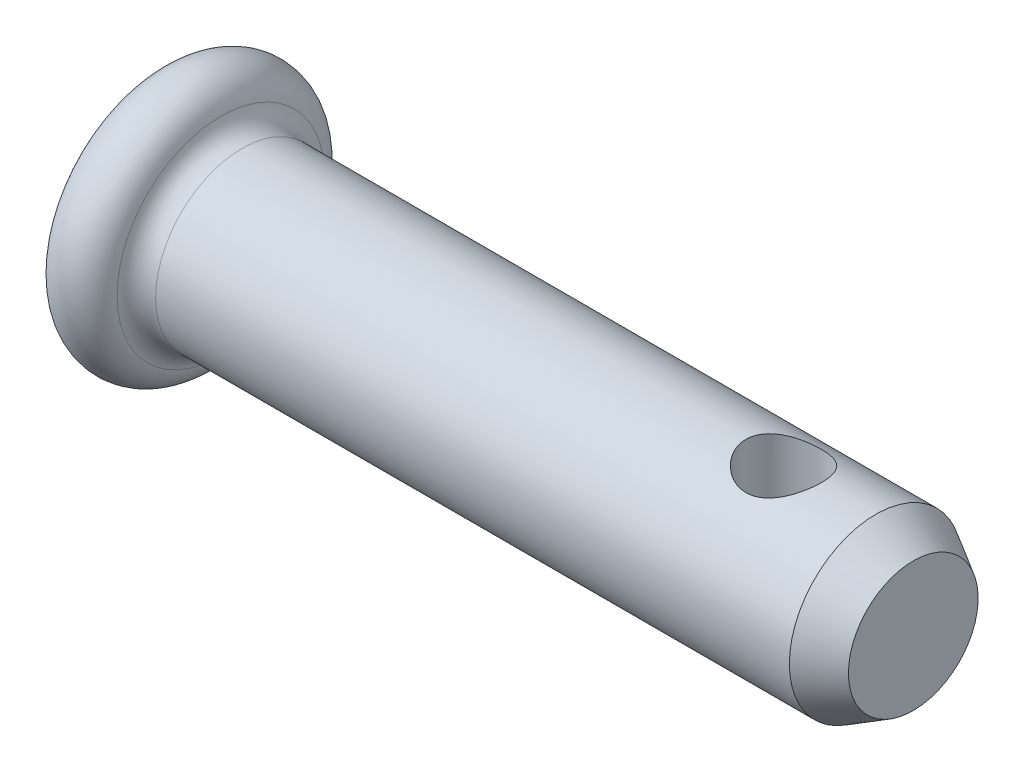
SolidWorks part; units mm, degrees
material "35钢"
ref_plane "前视" through (0, 0, 0) normal (0, 0, 1) x (1, 0, 0)
ref_plane "上视" through (0, 0, 0) normal (0, 1, 0) x (1, 0, 0)
ref_plane "右视" through (0, 0, 0) normal (1, 0, 0) x (0, 0, -1)
sketch "尺寸草图" plane through (0, 0, 0) normal (0, 0, 1) x (1, 0, 0)
  line L0 (0, 6) -> (0, 0)
  line L1 (0, 0) -> (16, 0)
  line L2 (16, 0) -> (19, 0) construction
  point P3 (0, 4)
  point P5 (1.5, 0)
  point P6 (0.5, 0)
  point P7 (15.5, 0)
  point P8 (3, 0)
  point P9 (0, 1.74)
sketch "草图1" plane through (0, 0, 0) normal (0, 0, 1) x (1, 0, 0)
  line L0 (0, 0) -> (10.7677, 0) construction
  line L1 (0, 0) -> (17.5, 0)
  line L2 (0, 0) -> (0, 2.25)
  line L4 (1.5, 2.25) -> (1.5, 2)
  line L5 (1.5, 2) -> (17.5, 2)
  line L6 (17.5, 2) -> (17.5, 0)
  arc A0 (0, 2.25) -> (1.5, 2.25) centre (0.75, 2.25) cw
revolve "基体-旋转" add sketch "草图1" angle 360 about L0
fillet "圆角1" radius 0.5 1 edges at (1.5, 0, 2)
chamfer "倒角1" distance 0.5 angle 60 1 edges at (17.5, 0, 2)
sketch "草图2" plane through (0, 0, 0) normal (0, 1, 0) x (1, 0, 0)
  circle A0 centre (14.5, 0) radius 0.87
extrude "切除-拉伸1" cut sketch "草图2" against normal mid plane 1000
equation "\"D4@草图1\" = \"K@尺寸草图\""
equation "\"D2@草图1\" = \"dk@尺寸草图\""
equation "\"D1@草图1\" = \"l@尺寸草图\""
equation "\"D3@草图1\" = \"d@尺寸草图\""
equation "\"D1@圆角1\" = \"r@尺寸草图\""
equation "\"D1@倒角1\" = \"c@尺寸草图\""
equation "\"D2@草图2\" = \"d1@尺寸草图\""
equation "\"lh@尺寸草图\" = \"l@尺寸草图\"-\"l-lh@尺寸草图\""
